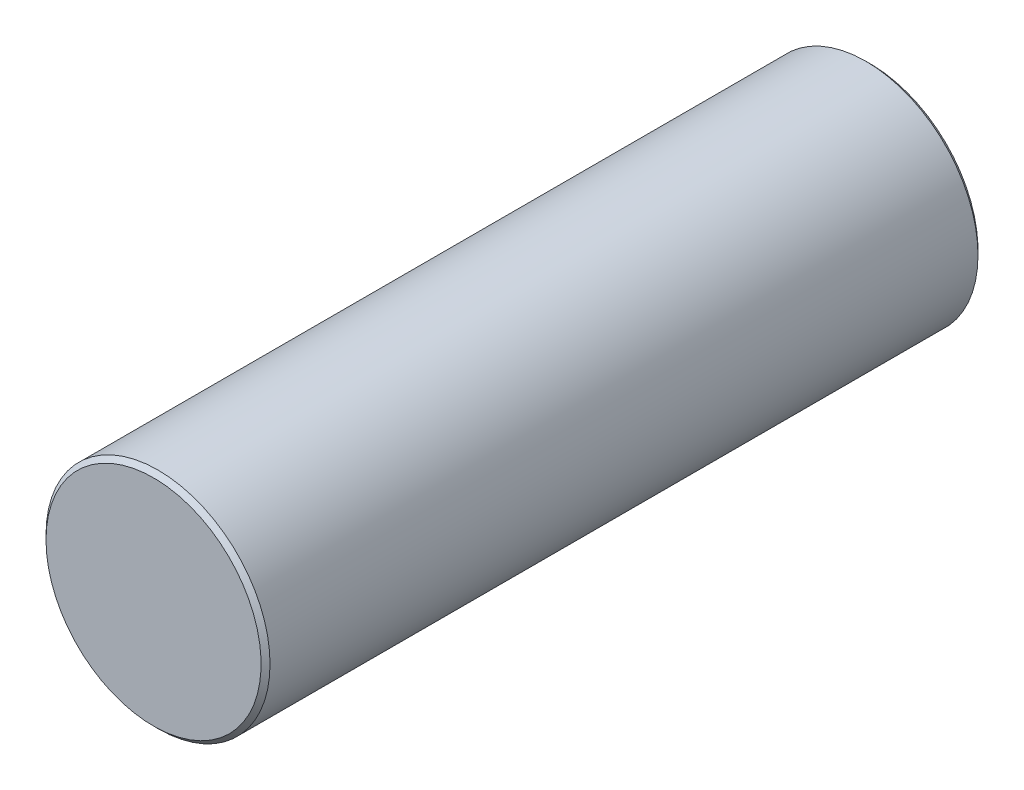
from build123d import *


with BuildPart() as part:
    # Sketch1 → Revolve1 (revolve)
    with BuildSketch(Plane.XZ, mode=Mode.PRIVATE) as revolve1_sk:
        Polygon((12, 80), (0, 80), (0, 0), (12, 0), (12.5, 0.5), (12.5, 79.5), align=None)
    revolve(revolve1_sk.sketch.rotate(Axis((0, 0, 80), (0, 0, -1)), 180), axis=Axis((0, 0, 80), (0, 0, -1)))


solid = part.part
